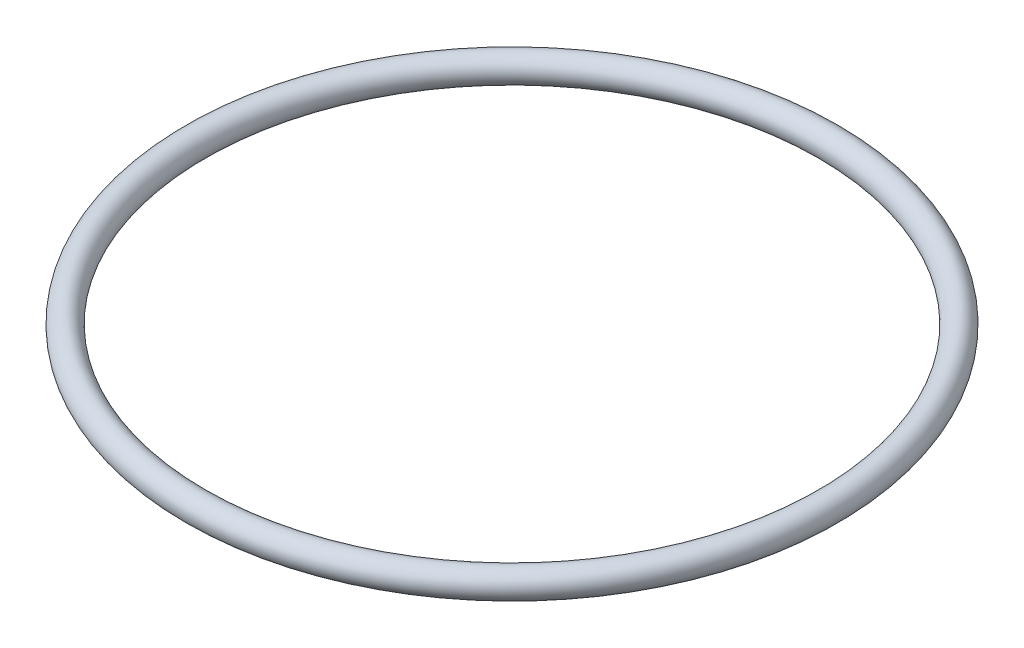
from build123d import *

# Parameters (mm, degrees)
SKETCH1_R = 1.765


with BuildPart() as part:
    # Sketch1 → Revolve1 (revolve)
    with BuildSketch(Plane.XY, mode=Mode.PRIVATE) as revolve1_sk:
        with Locations((41.25, 0)):
            Circle(SKETCH1_R)
    revolve(revolve1_sk.sketch.rotate(Axis((0, 6.392760857, 0), (0, -1, 0)), 90), axis=Axis((0, 6.392760857, 0), (0, -1, 0)))


solid = part.part
